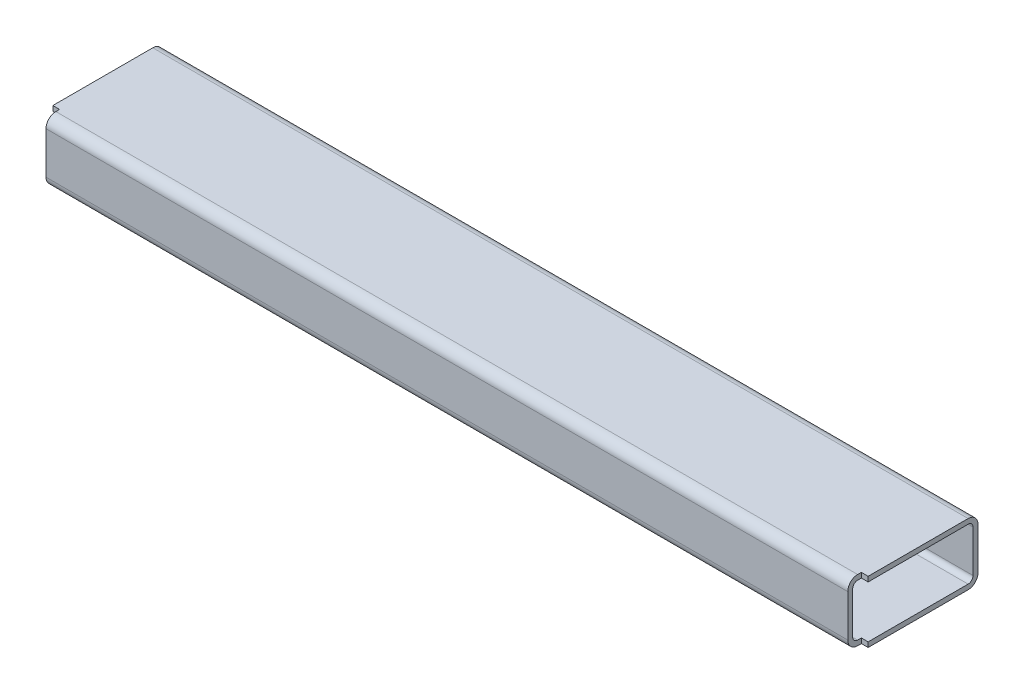
SolidWorks part; units mm, degrees
material "Q235B"
ref_plane "Front Plane" through (0, 0, 0) normal (0, 0, 1) x (1, 0, 0)
ref_plane "Top Plane" through (0, 0, 0) normal (0, 1, 0) x (1, 0, 0)
ref_plane "Right Plane" through (0, 0, 0) normal (1, 0, 0) x (0, 0, -1)
sketch "草图1" plane through (0, 0, 0) normal (0, 0, 1) x (1, 0, 0)
  line L0 (-660.5, 0) -> (660.5, 0)
  line L1 (0, 0) -> (0, 93.9196) construction
  dimension "D1" = 1321
other "Structural cold-formed rectangular hollow section (gb t6728-2002) 200×100×8(1)"
ref_plane "Plane1" through (-660.5, 0, 0) normal (1, 0, 0) x (0, 1, 0)
sketch "Sketch1" plane through (-660.5, 0, 0) normal (1, 0, 0) x (0, 1, 0)
  line L0 (-34, -92) -> (34, -92)
  line L1 (-42, -84) -> (-42, 84)
  line L2 (34, 92) -> (-34, 92)
  line L3 (42, 84) -> (42, -84)
  line L4 (-34, -100) -> (34, -100)
  line L5 (-50, -84) -> (-50, 84)
  line L6 (34, 100) -> (-34, 100)
  line L7 (50, 84) -> (50, -84)
  arc A0 (50, 84) -> (34, 100) centre (34, 84) ccw
  arc A1 (34, -100) -> (50, -84) centre (34, -84) ccw
  arc A2 (-50, -84) -> (-34, -100) centre (-34, -84) ccw
  arc A3 (-34, 100) -> (-50, 84) centre (-34, 84) ccw
  arc A4 (-34, 92) -> (-42, 84) centre (-34, 84) ccw
  arc A5 (42, 84) -> (34, 92) centre (34, 84) ccw
  arc A6 (34, -92) -> (42, -84) centre (34, -84) ccw
  arc A7 (-42, -84) -> (-34, -92) centre (-34, -84) ccw
  point P0 (0, 100)
  point P1 (50, 0)
  point P2 (0, -100)
  point P3 (-50, 0)
  point P4 (-50, 100)
  point P5 (50, 100)
  point P6 (50, -100)
  point P7 (-50, -100)
  point P8 (0, 0)
  point P33 (0, 0)
  dimension "D1" = 200
  dimension "D2" = 100
  dimension "D3" = 8
  dimension "D4" = 16
sketch "Sketch2" plane through (0, -50, 0) normal (0, -1, 0) x (1, 0, 0)
  line L0 (0, 100) -> (0, -100) construction
  line L1 (660.5, 100) -> (-660.5, 100) construction
  line L2 (660.5, -100) -> (-660.5, -100) construction
  line L3 (0, 0) -> (1400, 0) construction
  line L4 (-660.5, 100) -> (-649.5, 100)
  line L5 (-660.5, 100) -> (-660.5, 78)
  line L6 (-660.5, 78) -> (-649.5, 78)
  line L7 (-649.5, 100) -> (-649.5, 78)
  line L8 (-660.5, 0) -> (660.5, 0) construction
  line L9 (-649.5, -100) -> (-649.5, -78) construction
  line L10 (-660.5, -78) -> (-649.5, -78) construction
  line L11 (-660.5, -100) -> (-660.5, -78) construction
  line L12 (-660.5, -100) -> (-649.5, -100) construction
  dimension "D1" = 11
  dimension "D2" = 156
extrude "Cut-Extrude1" cut sketch "Sketch2" against normal through all
mirror "Mirror1" about plane through (0, 0, 0) normal (1, 0, 0) of "Cut-Extrude1"
